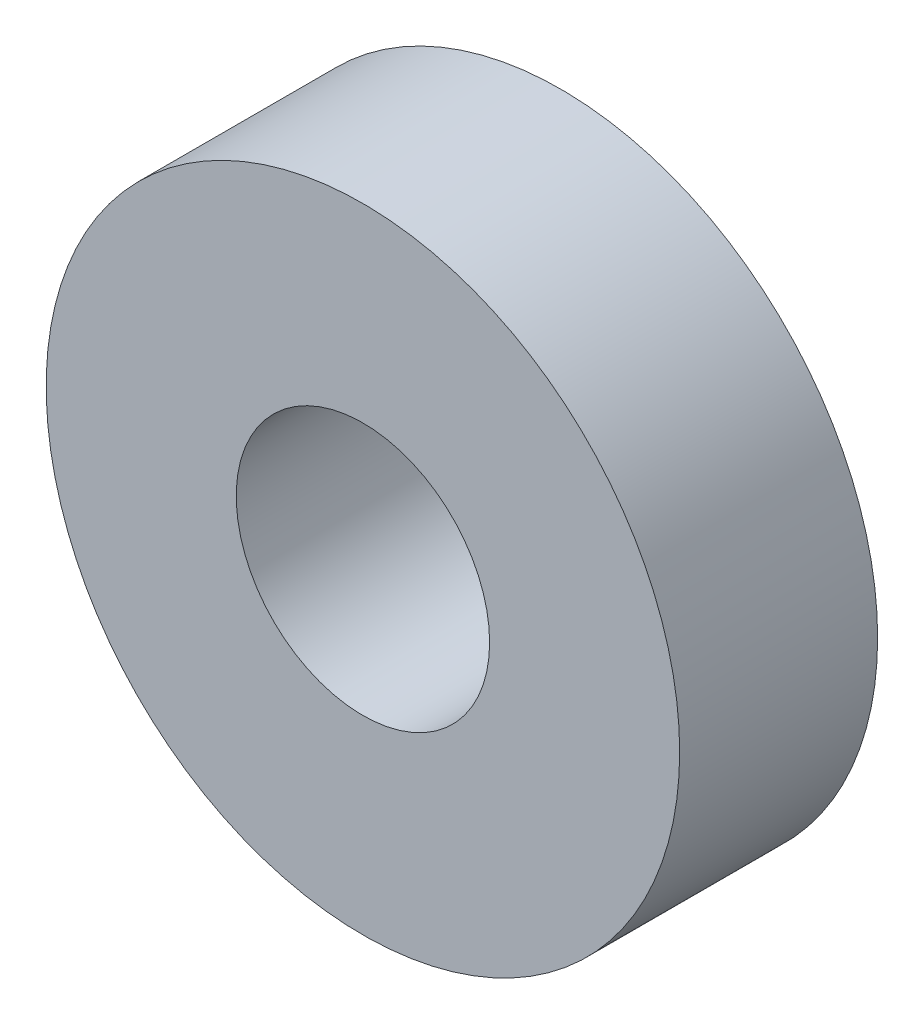
SolidWorks part; units mm, degrees
ref_plane "前视基准面" through (0, 0, 0) normal (0, 0, 1) x (1, 0, 0)
ref_plane "上视基准面" through (0, 0, 0) normal (0, 1, 0) x (1, 0, 0)
ref_plane "右视基准面" through (0, 0, 0) normal (1, 0, 0) x (0, 0, -1)
other "Configuration Table"
sketch "草图1" plane through (0, 0, 0) normal (0, 0, 1) x (1, 0, 0)
  circle A0 centre (0, 0) radius 8
  circle A1 centre (0, 0) radius 3.2
  point P0 (0, 0)
  dimension "D1" = 6.4
  dimension "D2" = 16
extrude "凸台-拉伸1" add sketch "草图1" against normal mid plane 5
